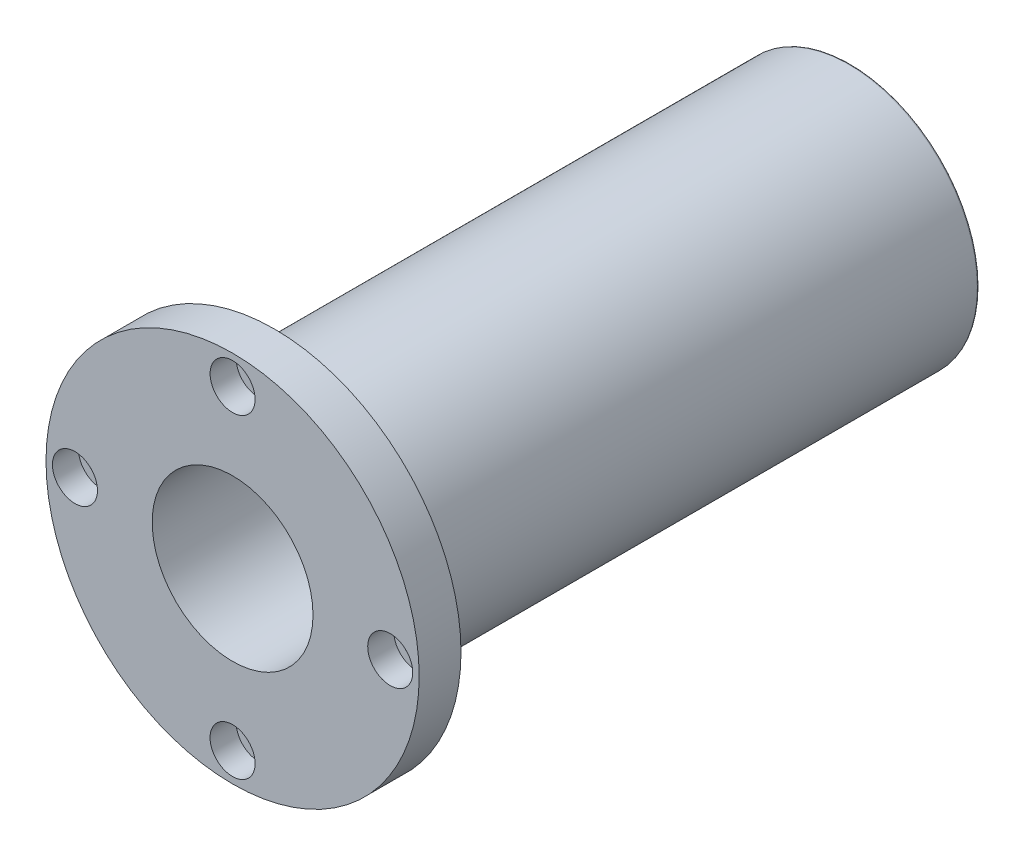
from build123d import *

# Parameters (mm, degrees)
SKETCH_1_W               = 179
SKETCH_1_H               = 15
FILLET_1_R               = 0.5
EXTRUDE_START            = 13
SKETCH_2_R               = 58
SKETCH_2_R_2             = 25
EXTRUDE_1_DEPTH          = 13
SKETCH_3_W               = 8.1
SKETCH_3_H               = 7
SKETCH_3_W_2             = 4.9
SKETCH_3_H_2             = 4.5
PATTERN_CIRCULAR_1_COUNT = 4


with BuildPart() as part:
    # 草图1 → 旋转1 (revolve)
    with BuildSketch(Plane(origin=(0, 0, 0), x_dir=(0, 0, -1), z_dir=(1, 0, 0)), mode=Mode.PRIVATE) as revolve_1_sk:
        with Locations((89.5, 32.5)):
            Rectangle(SKETCH_1_W, SKETCH_1_H)
    revolve(revolve_1_sk.sketch.rotate(Axis((0, 0, 0), (0, 0, -1)), 90), axis=Axis((0, 0, 0), (0, 0, -1)))

    # 圆角1
    fillet_1_edges = [part.edges().sort_by_distance(p)[0] for p in [
        (-40, 0, -179),
    ]]
    fillet(fillet_1_edges, radius=FILLET_1_R)

    # 草图2 → 凸台-拉伸1 (add)
    with BuildSketch(Plane.XY.offset(EXTRUDE_START)):
        with Locations(Location((0, 0, 0), (0, 0, 180))):
            Circle(SKETCH_2_R)
        Circle(SKETCH_2_R_2, mode=Mode.SUBTRACT)
    extrude(amount=-EXTRUDE_1_DEPTH)

    # 草图3 → 切除-旋转1 (revolve, cut)
    with BuildSketch(Plane(origin=(0, 0, 0), x_dir=(0, 0, -1), z_dir=(1, 0, 0)), mode=Mode.PRIVATE) as cut_revolve_1_sk:
        with Locations((-8.95, 52.5)):
            Rectangle(SKETCH_3_W, SKETCH_3_H)
        Polygon((-4.9, 56), (-13, 56), (-13, 49), (-4.9, 49), (-4.9, 53.5), align=None)
        with Locations((-2.45, 51.25)):
            Rectangle(SKETCH_3_W_2, SKETCH_3_H_2)
    cut_revolve_1 = revolve(cut_revolve_1_sk.sketch.rotate(Axis((0, 49, 0), (0, 0, -1)), 90), axis=Axis((0, 49, 0), (0, 0, -1)), mode=Mode.SUBTRACT)

    # 阵列(圆周)1: 切除-旋转1 ×4 about axis
    pattern_circular_1_axis = Axis((0, 0, 0), (0, 0, 1))
    for i in range(1, PATTERN_CIRCULAR_1_COUNT):
        add(cut_revolve_1.rotate(pattern_circular_1_axis, i * 360 / PATTERN_CIRCULAR_1_COUNT), mode=Mode.SUBTRACT)


solid = part.part
